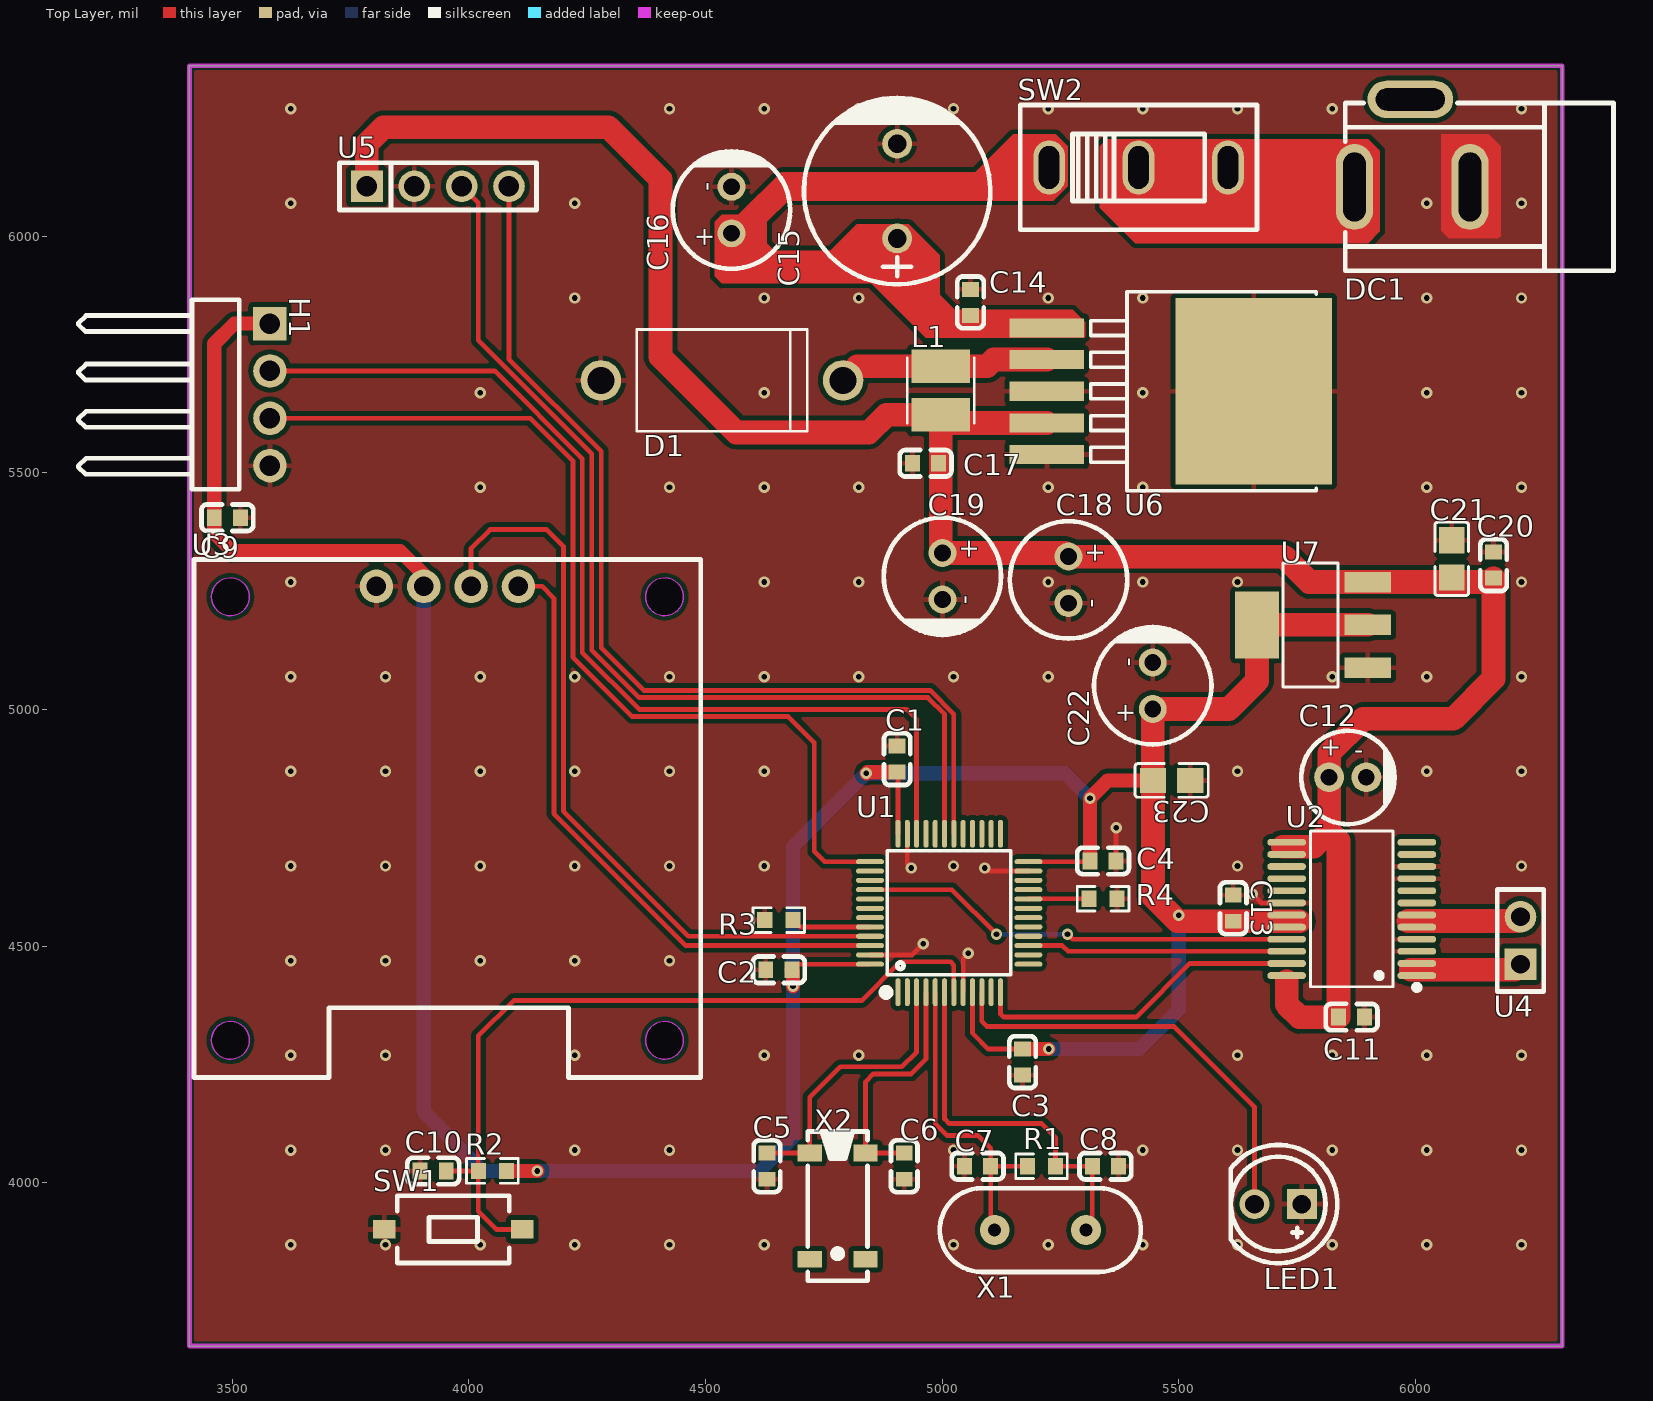
[diagram p0: Top Layer view]
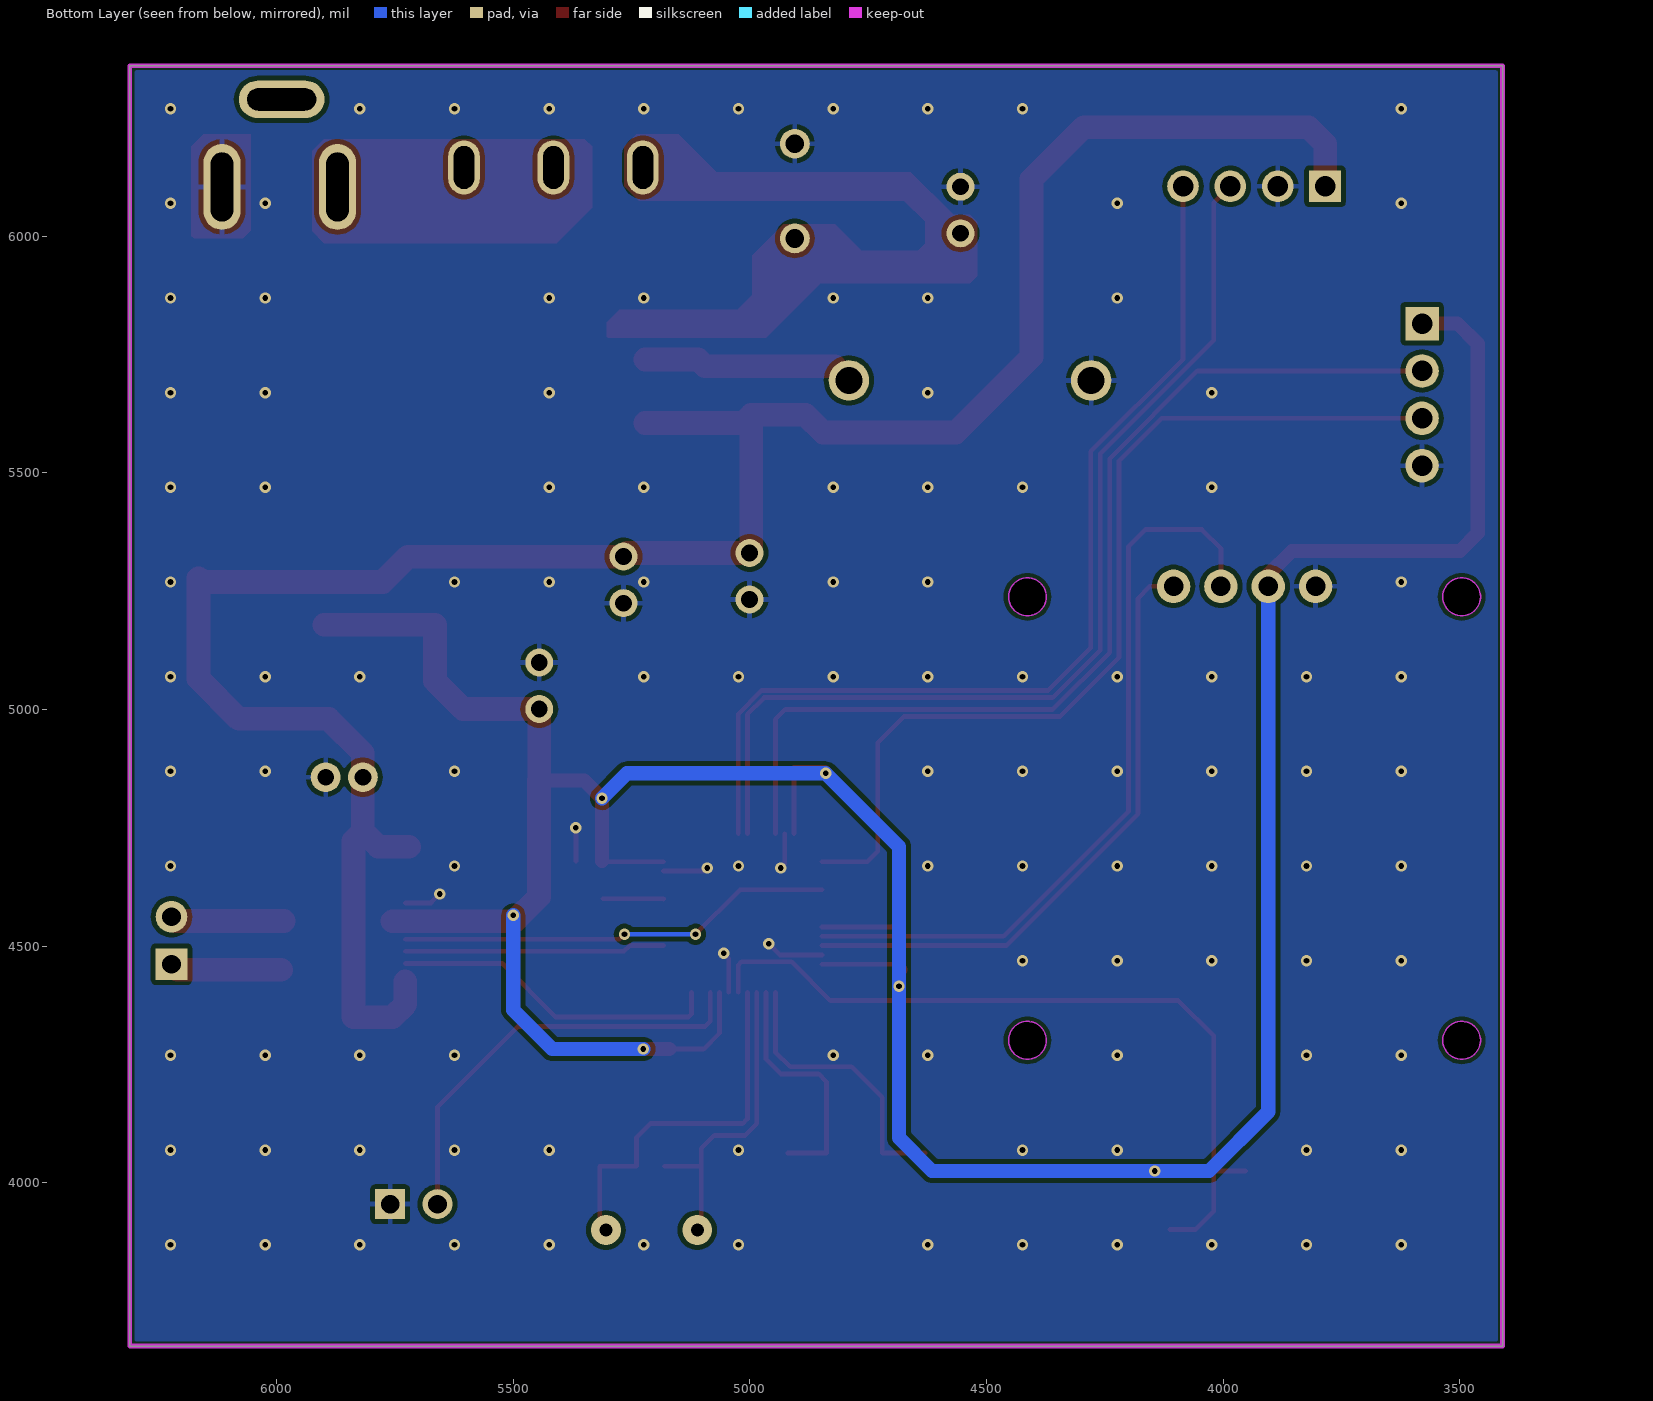
[diagram p1: Bottom Layer view, seen from below]
# Altium PCB MISC51997.pcbdoc
Units mil, origin at the board's own origin, x right, y up, seen from the top; angles counter-clockwise.
Board outline 2900 x 2705 mil, 2 copper layers (Top Layer, Bottom Layer), stack 62.206 mil thick; 43 components, 48 nets, 170 pads, 122 vias.

## Layer stack, top to bottom
Top Solder Mask Layer: solder mask 0.394, Dk 3.3
Top Layer: signal copper 1.379
Dielectric1: surface 59.449, FR4, Dk 4.5
Bottom Layer: signal copper 1.378
Bottom Solder Mask Layer: solder mask 0.394, Dk 3.3

## Board outline
3410,6360 3410,3655 6310,3655 6310,6360

## Design rules (kind name [scope] priority, off if disabled: settings)
BoardOutlineClearance copperThickness2oz_1 [All] p2 off: genericclearance=7.99 ignorepadtopadclearanceinfootprint=FALSE except(0: Arc-SplitContinuation Track-SplitContinuation SMDPad-SplitContinuation THPad-SplitContinuation Via-SplitContinuation Fill-SplitContinuation Region-SplitContinuation Poly-SplitContinuation Text-SplitContinuation Hole-SplitContinuation; 5.98: Arc-CutoutEdge SMDPad-CutoutEdge THPad-CutoutEdge Via-CutoutEdge Fill-CutoutEdge Region-CutoutEdge Text-CutoutEdge; 6.93: Hole-OutlineEdge Hole-CutoutEdge; 10: Poly-OutlineEdge Poly-CutoutEdge; 11.81: Arc-OutlineEdge Track-OutlineEdge SMDPad-OutlineEdge THPad-OutlineEdge Via-OutlineEdge Fill-OutlineEdge Region-OutlineEdge Text-OutlineEdge Track-CutoutEdge)
BoardOutlineClearance copperThickness1oz_1 [All] p4: genericclearance=4.02 ignorepadtopadclearanceinfootprint=FALSE except(0: Arc-SplitContinuation Track-SplitContinuation SMDPad-SplitContinuation THPad-SplitContinuation Via-SplitContinuation Fill-SplitContinuation Region-SplitContinuation Poly-SplitContinuation Text-SplitContinuation Hole-SplitContinuation; 6: SMDPad-CutoutEdge THPad-CutoutEdge Via-CutoutEdge Fill-CutoutEdge Region-CutoutEdge Text-CutoutEdge; 6.93: Hole-OutlineEdge Hole-CutoutEdge; 10: Poly-OutlineEdge Poly-CutoutEdge; 11.8: Arc-OutlineEdge Track-OutlineEdge SMDPad-OutlineEdge THPad-OutlineEdge Via-OutlineEdge Fill-OutlineEdge Region-OutlineEdge Text-OutlineEdge; 11.81: Arc-CutoutEdge Track-CutoutEdge)
Clearance copperThickness2oz [All] p1 off: gap=7.99 ignorepadtopadclearanceinfootprint=FALSE except(5.98: SMDPad-Track SMDPad-SMDPad THPad-Track SMDPad-THPad THPad-THPad Track-Via SMDPad-Via THPad-Via Via-Via Fill-Track Region-Track Fill-SMDPad Region-SMDPad Fill-THPad Region-THPad Fill-Via Region-Via Fill-Fill Fill-Region Region-Region Arc-Track Arc-SMDPad Arc-THPad Arc-Via Fill-Arc Region-Arc Arc-Arc Text-Track SMDPad-Text Text-THPad Text-Via Fill-Text Region-Text Arc-Text Text-Text; 6.93: Hole-Track Hole-SMDPad Hole-THPad Hole-Via Fill-Hole Region-Hole Hole-Arc Hole-Text; 10: Poly-Track Poly-SMDPad Poly-THPad Poly-Via Poly-Fill Poly-Region Poly-Poly Poly-Arc Poly-Text Poly-Hole)
Clearance copperThickness1oz [All] p3: gap=4.02 ignorepadtopadclearanceinfootprint=FALSE except(5.98: SMDPad-Track SMDPad-SMDPad THPad-Track SMDPad-THPad THPad-THPad Track-Via SMDPad-Via THPad-Via Via-Via Fill-Track Region-Track Fill-SMDPad Region-SMDPad Fill-THPad Region-THPad Fill-Via Region-Via Fill-Fill Fill-Region Region-Region; 6: Arc-Track Arc-SMDPad Arc-THPad Arc-Via Fill-Arc Region-Arc Arc-Arc Text-Track SMDPad-Text Text-THPad Text-Via Fill-Text Region-Text Arc-Text Text-Text; 6.93: Hole-Track Hole-SMDPad Hole-THPad Hole-Via Fill-Hole Region-Hole Hole-Arc Hole-Text; 10: Poly-Track Poly-SMDPad Poly-THPad Poly-Via Poly-Fill Poly-Region Poly-Poly Poly-Arc Poly-Text Poly-Hole)
Creepage creepage [All] p1: checkdistance=0 ignoreinternallayers=TRUE applytopolygonpour=TRUE
DiffPairsRouting differentialPair [All] p1: maxlimit=6 minlimit=6 mostfreqgap=6 toplayer_minwidth=5 toplayer_prefwidth=10 toplayer_maxwidth=100 toplayer_mingap=6 toplayer_prefgap=6 toplayer_maxgap=6 bottomlayer_minwidth=5 bottomlayer_prefwidth=10 bottomlayer_maxwidth=100 bottomlayer_mingap=6 bottomlayer_prefgap=6 bottomlayer_maxgap=6 maxuncoupledlength=10
HoleToHoleClearance otherClearance [All] p1: gap=11.81 allowstackedmicrovias=TRUE
Length netLength [All] p1: minlimit=0 maxlimit=0
MatchedLengths netLengthTolerance [All] p1: tolerance=1000
PasteMaskExpansion pasteMaskExpansion [All] p1: expansion=0
PlaneConnect innerPlane [All] p1: planeconnectstyle=Relief reliefexpansion=20 reliefentries=4 reliefconductorwidth=10 reliefairgap=10
PolygonConnect copperRegion [(InNet('GND'))] p1: connectstyle=Relief reliefconductorwidth=10 reliefentries=4 polygonreliefangle="90 Angle" airgapwidth=10 via.connectstyle=Relief via.reliefconductorwidth=10 via.reliefentries=4 via.polygonreliefangle="90 Angle" via.airgapwidth=10
RoutingVias viaSize [All] p1: holewidth=12.01 width=24.02 viastyle="Through Hole" minholewidth=11.81 minwidth=19.68 maxholewidth=248.03 maxwidth=393.7
SolderMaskExpansion solderMaskExpansion [IsVia] p1: expansion=-1000 istentingtop=TRUE
SolderMaskExpansion solderMaskExpansion [All] p2: expansion=2 istentingtop=FALSE
Width copperThickness2oz_2 [All] p1 off: maxlimit=100 minlimit=8 preferedwidth=10
Width copperThickness1oz_2 [All] p2: maxlimit=100 minlimit=5 preferedwidth=10

## Components (designator, comment, footprint, x,y, rotation, side; value= is the part's Value field where it differs from the comment)
C1 "100nF" C0603 4905,4895 r270 top
C2 "100nF" C0603 4655,4450 r0 top
C3 "100nF" C0603 5170,4255 r90 top
C4 "100nF" C0603 5340,4680 r180 top
C5 "20pF" C0603 4630,4035 r270 top
C6 "20pF" C0603 4920,4035 r270 top
C7 "20pF" C0603 5075,4035 r180 top
C8 "20pF" C0603 5345,4035 r0 top
C9 "100nF" C0603 3490,5405 r180 top
C10 "1uF" C0603 3925,4025 r0 top
C11 "100nF" C0603 5865,4350 r180 top
C12 "10uF" CAP-TH_BD5.0-P2.00-D0.5-FD-A 5856.9,4856.84 r0 top
C13 "100nF" C0603 5615,4580 r270 top
C14 "100nF" C0603 5060,5860 r270 top
C15 "220uF" CAP-TH_BD10.0-P5.00-D1.0-FD 4905,6095 r90 top
C16 "100uF" CAP-TH_BD6.3-P2.50-D0.5-FD 4555,6055 r90 top
C17 "100nF" C0603 4965,5520 r0 top
C18 "220uF" CAP-TH_BD6.3-P2.50-D0.5-FD_DXW025M227E112S1AA 5267.14,5273.67 r270 top
C19 "100uF" CAP-TH_BD6.3-P2.50-D0.5-FD 5000.64,5281.38 r270 top
C20 "100nF" C0603 6165,5305 r270 top
C21 "10uF" C0805 6076.65,5317.95 r270 top
C22 "100uF" CAP-TH_BD6.3-P2.50-D0.5-FD 5445,5050 r90 top
C23 "10uF" C0805 5485,4850 r180 top
D1 "1N5824" DO-201AD_BD5.3-L9.0-P13.00-D1.3-RD 4535,5695 r180 top
DC1 "DC005" DC-IN-TH_DC005 5993.2,6196.3 r180 top
H1 "PZ254R-11-04P" HDR-TH_4P-P2.54-H-M-W10.4 3580,5665 r270 top
L1 "33uH" IND-SMD_L3.5-W3.0 4997.14,5673.67 r90 top
LED1 "BL-BUB1V4V-AT" LED-TH_BD5.8-P2.54-FD_RED 5710,3955 r180 top
R1 "1MΩ" R0603 5210,4035 r180 top
R2 "10kΩ" R0603 4050,4025 r0 top
R3 "100kΩ" R0603 4655,4555 r0 top
R4 "100kΩ" R0603 5340,4600 r180 top
SW1 "TS-1101-C-W" SW-SMD_L6.0-W3.3-LS8.0_TS-1101-C-W 3967.28,3901.5 r0 top
SW2 "SS12D10G4" SW-TH_3P-P4.80-HX-SS12D10G4 5415.01,6145.01 r0 top
U1 "STM32F103C8T6" LQFP-48_L7.0-W7.0-P0.50-LS9.0-BL 5015,4570 r0 top
U2 "TB6612FNG" SSOP-24_L8.4-W5.8-P0.65-LS7.8-BL 5865.4,4578.48 r90 top
U3 "HS96L03W2C03" OLED-TH_L27.8-W27.2-P2.54_C9900033791 3955,5260 r0 top
U4 "2.54-1*2P母" HDR-TH_2P-P2.54-V-F 6221.9,4511.84 r90 top
U5 "2.54-1*4P母" HDR-TH_4P-P2.54-V-F 3935,6105 r0 top
U6 "LM2596SX-5.0-JSM" TO-263-5_L10.0-W8.4-P1.70-LS15.3-BR 5439.86,5672.17 r180 top
U7 "AMS1117-3.3" SOT-223-3_L6.5-W3.4-P2.30-LS7.0-BR 5782.28,5178.58 r0 top
X1 "8MHz" OSC-TH_L10.0-W4.5-P5.00 5207.58,3900.2 r90 top
X2 "32.768kHz" MC-306_4P-L8.0-W3.2-P5.5-BL 4779.33,3950.67 r270 top

## Footprints (in the part's own frame and the unit in brackets; to place one, negate y for a bottom-side part, rotate by r counter-clockwise, add the part's x,y. Pads: shape width x height; smd on the part's side, far side on the other; paste and mask are expansions set on the pad)
C0603 [mm]
  rect 0.8x0.9 smd: 1(-0.7,0) 2(0.7,0)
  silkscreen extent -1.39,-0.71 1.39,0.71
C0805 [mm]
  rect 1.41x1.35 smd paste-100 mask+0.051: 1(-1,0) 2(1,0)
  silkscreen extent -1.96,-0.9 1.96,0.9
CAP-TH_BD5.0-P2.00-D0.5-FD-A [mm]
  round 1.6 hole 0.9 paste+0 mask+0.05: 1(-1,0) 2(1,0)
  silkscreen extent -2.49,-2.52 2.6,2.49
CAP-TH_BD6.3-P2.50-D0.5-FD [mm]
  round 1.5 hole 0.9 paste+0 mask+0.05: 1(-1.25,0) 2(1.25,0)
  silkscreen extent -3.15,-3.15 3.21,3.15
CAP-TH_BD6.3-P2.50-D0.5-FD_DXW025M227E112S1AA [mm]
  round 1.5 hole 0.9 paste+0 mask+0.05: 1(-1.25,0) 2(1.25,0)
  silkscreen extent -3.15,-3.15 3.15,3.15
CAP-TH_BD10.0-P5.00-D1.0-FD [mm]
  round 1.6 hole 1: 1(-2.54,0) 2(2.54,0)
  silkscreen extent -5,-5 5.08,5
DC-IN-TH_DC005 [mm]
  oval 2x4.6 hole 1.2 slot 3.7 at 90 deg: 1(3.1,2.35) 2(-3.1,2.35)
  oval 4.6x2 hole 1.2 slot 3.7 at 0 deg: 3(0.1,-2.35)
  silkscreen extent -10.8,-2.15 3.6,6.85
DO-201AD_BD5.3-L9.0-P13.00-D1.3-RD [mm]
  round 2.175 hole 1.45: 1(-6.5,0) 2(6.5,0)
  silkscreen extent -4.58,-2.73 4.58,2.73
HDR-TH_2P-P2.54-V-F [mm]
  rect 1.7x1.7 hole 1: 1(-1.27,0)
  round 1.7 hole 1: 2(1.27,0)
  silkscreen extent -2.74,-1.25 2.74,1.25
HDR-TH_4P-P2.54-H-M-W10.4 [mm]
  rect 1.8x1.8 hole 1.1: 1(-3.81,0)
  round 1.8 hole 1.1: 2(-1.27,0) 3(1.27,0) 4(3.81,0)
  silkscreen extent -5.09,-10.27 5.07,-1.65
HDR-TH_4P-P2.54-V-F [mm]
  rect 1.7x1.7 hole 1.1: 1(-3.81,0)
  round 1.7 hole 1.1: 2(-1.27,0) 3(1.27,0) 4(3.81,0)
  silkscreen extent -5.29,-1.27 5.29,1.27
IND-SMD_L3.5-W3.0 [mm]
  rect 1.8x3.12 smd: 1(1.303,0) 2(-1.303,0)
  silkscreen extent -1.75,-1.8 1.75,1.8
LED-TH_BD5.8-P2.54-FD_RED [mm]
  rect 1.6x1.6 hole 1: 1(-1.27,0)
  round 1.6 hole 1: 2(1.27,0)
  silkscreen extent -3.17,-3.17 2.54,3.17
LQFP-48_L7.0-W7.0-P0.50-LS9.0-BL [mm]
  oval 0.27x1.5 smd paste+0 mask+0.05: 1(-2.75,-4.25) 2(-2.25,-4.25) 3(-1.75,-4.25) 4(-1.25,-4.25) 5(-0.75,-4.25) 6(-0.25,-4.25) 7(0.25,-4.25) 8(0.75,-4.25) 9(1.25,-4.25) 10(1.75,-4.25) 11(2.25,-4.25) 12(2.75,-4.25) 25(2.75,4.25) 26(2.25,4.25) 27(1.75,4.25) 28(1.25,4.25) 29(0.75,4.25) 30(0.25,4.25) 31(-0.25,4.25) 32(-0.75,4.25) 33(-1.25,4.25) 34(-1.75,4.25) 35(-2.25,4.25) 36(-2.75,4.25)
  oval 1.5x0.27 smd paste+0 mask+0.05: 13(4.25,-2.75) 14(4.25,-2.25) 15(4.25,-1.75) 16(4.25,-1.25) 17(4.25,-0.75) 18(4.25,-0.25) 19(4.25,0.25) 20(4.25,0.75) 21(4.25,1.25) 22(4.25,1.75) 23(4.25,2.25) 24(4.25,2.75) 37(-4.25,2.75) 38(-4.25,2.25) 39(-4.25,1.75) 40(-4.25,1.25) 41(-4.25,0.75) 42(-4.25,0.25) 43(-4.25,-0.25) 44(-4.25,-0.75) 45(-4.25,-1.25) 46(-4.25,-1.75) 47(-4.25,-2.25) 48(-4.25,-2.75)
  silkscreen extent -3.59,-4.46 3.3,3.34
MC-306_4P-L8.0-W3.2-P5.5-BL [mm]
  rect 0.9x1.3 smd: 1(-2.85,-1.5) 2(2.85,-1.5) 3(2.85,1.5) 4(-2.85,1.5)
  silkscreen extent -4,-1.6 4,1.6
OLED-TH_L27.8-W27.2-P2.54_C9900033791 [mm]
  round 1.8 hole 1.05 paste+0 mask+0.05: 1(-3.81,0) 2(-1.27,0) 3(1.27,0) 4(3.81,0)
  Board Outline Layer circle w0.003: c-11.65,-0.56 r1.016
  Board Outline Layer circle w0.003: c11.65,-0.56 r1.016
  Board Outline Layer circle w0.003: c-11.65,-24.36 r1.016
  Board Outline Layer circle w0.003: c11.65,-24.36 r1.016
  Board Outline Layer region: -10.634,-0.56 -10.735,-1.001 -11.016,-1.354 -11.424,-1.551 -11.876,-1.551 -12.283,-1.354 -12.565,-1.001 -12.666,-0.56 -12.666,-0.56 -12.565,-0.119 -12.283,0.234 -11.876,0.431 -11.424,0.431 -11.016,0.234 -10.735,-0.119 -10.634,-0.56
  Board Outline Layer region: -10.634,-0.56 -10.643,-0.698 -10.672,-0.834 -10.718,-0.965 -10.782,-1.088 -10.862,-1.201 -10.956,-1.303 -11.064,-1.39 -11.183,-1.462 -11.31,-1.517 -11.443,-1.555 -11.581,-1.574 -11.719,-1.574 -11.857,-1.555 -11.99,-1.517 -12.117,-1.462 -12.236,-1.39 -12.343,-1.303 -12.438,-1.201 -12.518,-1.088 -12.582,-0.965 -12.628,-0.834 -12.656,-0.698 -12.666,-0.56 -12.656,-0.422 -12.628,-0.286 -12.582,-0.155 -12.518,-0.032 -12.438,0.081 -12.343,0.183 -12.236,0.27 -12.117,0.342 -11.99,0.397 -11.857,0.435 -11.719,0.454 -11.581,0.454 -11.443,0.435 -11.31,0.397 -11.183,0.342 -11.064,0.27 -10.956,0.183 -10.862,0.081 -10.782,-0.032 -10.718,-0.155 -10.672,-0.286 -10.643,-0.422
  Board Outline Layer region: 12.666,-0.56 12.565,-1.001 12.283,-1.354 11.876,-1.551 11.424,-1.551 11.017,-1.354 10.735,-1.001 10.634,-0.56 10.634,-0.56 10.735,-0.119 11.017,0.234 11.424,0.431 11.876,0.431 12.283,0.234 12.565,-0.119 12.666,-0.56
  Board Outline Layer region: 12.666,-0.56 12.657,-0.698 12.628,-0.834 12.582,-0.965 12.518,-1.088 12.438,-1.201 12.343,-1.303 12.236,-1.39 12.117,-1.462 11.99,-1.517 11.857,-1.555 11.719,-1.574 11.581,-1.574 11.443,-1.555 11.31,-1.517 11.183,-1.462 11.064,-1.39 10.957,-1.303 10.862,-1.201 10.782,-1.088 10.718,-0.965 10.672,-0.834 10.643,-0.698 10.634,-0.56 10.643,-0.422 10.672,-0.286 10.718,-0.155 10.782,-0.032 10.862,0.081 10.957,0.183 11.064,0.27 11.183,0.342 11.31,0.397 11.443,0.435 11.581,0.454 11.719,0.454 11.857,0.435 11.99,0.397 12.117,0.342 12.236,0.27 12.343,0.183 12.438,0.081 12.518,-0.032 12.582,-0.155 12.628,-0.286 12.657,-0.422
  Board Outline Layer region: -10.634,-24.36 -10.735,-24.801 -11.016,-25.154 -11.424,-25.35 -11.876,-25.35 -12.283,-25.154 -12.565,-24.801 -12.666,-24.36 -12.666,-24.36 -12.565,-23.919 -12.283,-23.566 -11.876,-23.369 -11.424,-23.369 -11.016,-23.566 -10.735,-23.919 -10.634,-24.36
  Board Outline Layer region: -10.634,-24.36 -10.643,-24.498 -10.672,-24.634 -10.718,-24.765 -10.782,-24.888 -10.862,-25.001 -10.956,-25.102 -11.064,-25.19 -11.183,-25.262 -11.31,-25.317 -11.443,-25.355 -11.581,-25.374 -11.719,-25.374 -11.857,-25.355 -11.99,-25.317 -12.117,-25.262 -12.236,-25.19 -12.343,-25.102 -12.438,-25.001 -12.518,-24.888 -12.582,-24.765 -12.628,-24.634 -12.656,-24.498 -12.666,-24.36 -12.656,-24.222 -12.628,-24.086 -12.582,-23.955 -12.518,-23.832 -12.438,-23.719 -12.343,-23.617 -12.236,-23.53 -12.117,-23.458 -11.99,-23.403 -11.857,-23.365 -11.719,-23.346 -11.581,-23.346 -11.443,-23.365 -11.31,-23.403 -11.183,-23.458 -11.064,-23.53 -10.956,-23.617 -10.862,-23.719 -10.782,-23.832 -10.718,-23.955 -10.672,-24.086 -10.643,-24.222
  Board Outline Layer region: 12.666,-24.36 12.565,-24.801 12.283,-25.154 11.876,-25.35 11.424,-25.35 11.017,-25.154 10.735,-24.801 10.634,-24.36 10.634,-24.36 10.735,-23.919 11.017,-23.566 11.424,-23.369 11.876,-23.369 12.283,-23.566 12.565,-23.919 12.666,-24.36
  Board Outline Layer region: 12.666,-24.36 12.657,-24.498 12.628,-24.634 12.582,-24.765 12.518,-24.888 12.438,-25.001 12.343,-25.102 12.236,-25.19 12.117,-25.262 11.99,-25.317 11.857,-25.355 11.719,-25.374 11.581,-25.374 11.443,-25.355 11.31,-25.317 11.183,-25.262 11.064,-25.19 10.957,-25.102 10.862,-25.001 10.782,-24.888 10.718,-24.765 10.672,-24.634 10.643,-24.498 10.634,-24.36 10.643,-24.222 10.672,-24.086 10.718,-23.955 10.782,-23.832 10.862,-23.719 10.957,-23.617 11.064,-23.53 11.183,-23.458 11.31,-23.403 11.443,-23.365 11.581,-23.346 11.719,-23.346 11.857,-23.365 11.99,-23.403 12.117,-23.458 12.236,-23.53 12.343,-23.617 12.438,-23.719 12.518,-23.832 12.582,-23.955 12.628,-24.086 12.657,-24.222
  Multi-Layer board cut-out: -10.634,-0.56 -10.735,-1.001 -11.016,-1.354 -11.424,-1.551 -11.876,-1.551 -12.283,-1.354 -12.565,-1.001 -12.666,-0.56 -12.666,-0.56 -12.565,-0.119 -12.283,0.234 -11.876,0.431 -11.424,0.431 -11.016,0.234 -10.735,-0.119 -10.634,-0.56
  Multi-Layer board cut-out: 12.666,-0.56 12.565,-1.001 12.283,-1.354 11.876,-1.551 11.424,-1.551 11.017,-1.354 10.735,-1.001 10.634,-0.56 10.634,-0.56 10.735,-0.119 11.017,0.234 11.424,0.431 11.876,0.431 12.283,0.234 12.565,-0.119 12.666,-0.56
  Multi-Layer board cut-out: -10.634,-24.36 -10.735,-24.801 -11.016,-25.154 -11.424,-25.35 -11.876,-25.35 -12.283,-25.154 -12.565,-24.801 -12.666,-24.36 -12.666,-24.36 -12.565,-23.919 -12.283,-23.566 -11.876,-23.369 -11.424,-23.369 -11.016,-23.566 -10.735,-23.919 -10.634,-24.36
  Multi-Layer board cut-out: 12.666,-24.36 12.565,-24.801 12.283,-25.154 11.876,-25.35 11.424,-25.35 11.017,-25.154 10.735,-24.801 10.634,-24.36 10.634,-24.36 10.735,-23.919 11.017,-23.566 11.424,-23.369 11.876,-23.369 12.283,-23.566 12.565,-23.919 12.666,-24.36
  silkscreen extent -13.6,-26.36 13.6,1.44
OSC-TH_L10.0-W4.5-P5.00 [mm]
  round 1.6 hole 0.7: 1(0,2.45) 2(0,-2.45)
  silkscreen extent -2.25,-5.39 2.25,5.39
R0603 [mil]
  rect 31.75x34.02 smd paste-3937.01 mask+2: 1(-29.66,0) 2(29.66,0)
  silkscreen extent -55,-26 55,26
SOT-223-3_L6.5-W3.4-P2.30-LS7.0-BR [mm]
  rect 2.5x1.1 smd: 1(2.97,-2.3) 2(2.97,0) 3(2.97,2.3)
  rect 2.34x3.6 smd: 4(-2.97,0)
  silkscreen extent -1.57,-3.33 1.37,3.33
SSOP-24_L8.4-W5.8-P0.65-LS7.8-BL [mil]
  oval 14.33x81.97 smd: 1(-140.75,-137.44) 2(-115.16,-137.44) 3(-89.57,-137.44) 4(-63.98,-137.44) 5(-38.39,-137.44) 6(-12.79,-137.44) 7(12.8,-137.44) 8(38.39,-137.44) 9(63.98,-137.44) 10(89.57,-137.44) 11(115.16,-137.44) 12(140.75,-137.44) 13(140.75,137.44) 14(115.16,137.44) 15(89.57,137.44) 16(63.98,137.44) 17(38.39,137.44) 18(12.8,137.44) 19(-12.79,137.44) 20(-38.39,137.44) 21(-63.98,137.44) 22(-89.57,137.44) 23(-115.16,137.44) 24(-140.75,137.44)
  silkscreen extent -172,-143 164,87
SW-SMD_L6.0-W3.3-LS8.0_TS-1101-C-W [mm]
  rect 1.2x1 smd: 1(-3.7,0) 2(3.7,0)
  silkscreen extent -3,-1.8 3,1.8
SW-TH_3P-P4.80-HX-SS12D10G4 [mm]
  oval 1.7x2.9 hole 1.1 slot 2.3 at 90 deg paste+0 mask+0.05: 1(-4.8,0) 2(0,0) 3(4.8,0)
  silkscreen extent -6.35,-3.35 6.35,3.35
TO-263-5_L10.0-W8.4-P1.70-LS15.3-BR [mm]
  rect 4x1.02 smd: 1(5.55,-3.4) 2(5.55,-1.7) 3(5.55,0) 4(5.55,1.7) 5(5.55,3.4)
  rect 8.4x10 smd: 6(-5.55,0)
  silkscreen extent -8.91,-5.33 3.2,5.33

## Via types
v1: diameter 24.02, hole 12, Top Layer to Bottom Layer, 122 vias

## Nets (pads, with @x,y where several pads share a name; then routed paths per layer and width w, separated by ;. In a path a pad name is that pad's centre, name@x,y a point inside that pad or via, vN(x,y) a via of type N, cw(c..) or ccw(c..) an arc to the next point about the centre after c; other vN are vias at no path point)
$1N2: DC1.1 SW2.2 SW2.3
$1N10: D1.1 L1.1 U6.2 | length 448.7
  Top Layer w50: D1.1 4820.88,5724.97 L1.1 5094.97,5724.97 5109.1,5739.1 U6.2
+5V: C11.2 C12.1 C17.2 C18.1 C19.1 C20.2 C21.2 L1.2 U2.13 U2.14 U2.24 U5.1 U6.4 U7.3 | length 5007.8
  Top Layer w50: U5.1 3784.64,6105.36 3784.64,6194.64 3820,6230 4295,6230 4405,6120 4405,5745 4565,5585 4845,5585 4882.37,5622.37 L1.2 ; U6.4 5014.27,5605.24 L1.2 ; 5720,4710 5785,4710 5817.53,4742.53 ; 5727.96,4425.18 5727.96,4377.04 5755,4350 C11.2 5837.44,4722.63 5817.53,4742.53 ; L1.2 4997.14,5334.09 C19.1 5259.43,5330.59 C18.1 5722.12,5322.88 5775.87,5269.13 U7.3 6156.69,5269.13 C20.2 6165,5065 6080,4980 5890,4980 5817.53,4907.53 C12.1 5817.53,4742.53
AO1: U2.1 U2.2 U4.1 | length 236.8
  Top Layer w50: 5990,4450 6210.07,4450 U4.1
AO2: U2.5 U2.6 U4.2 | length 240.5
  Top Layer w50: 5985,4553.14 6213.2,4553.14 U4.2
BAT: C14.2 C15.1 C16.1 SW2.1 U6.1
BOOT0: R3.2 U1.44 | length 169
  Top Layer w10: R3.2 4699.19,4540.47 U1.44
BOOT1: R4.2 U1.20 | length 128.2
  Top Layer w10: U1.20 5182.79,4600 R4.2
GND: C1.1 C2.1 C3.1 C4.1 C5.2 C6.2 C7.2 C8.2 C9.1 C10.1 C11.1 C12.2 C13.1 C14.1 C15.2 C16.2 C17.1 C18.2 C19.2 C20.1 C21.1 C22.2 C23.1 D1.2 DC1.2 H1.4 LED1.1 R3.1 R4.1 SW1.1 U1.8 U1.23 U1.35 U1.47 U2.3 U2.4 U2.9 U2.10 U2.18 U3.1 U5.2 U6.3 U6.5 U6.6 U7.1 | length 530.3
  Top Layer w10: U1.47 4936.42,4481.42 v1(4960,4505) ; U1.35 4926.42,4673.58 v1(4935,4665) ; U1.8 5044.53,4474.53 v1(5055,4485) ; v1(5090,4665) 5096.42,4658.58 U1.23 ; C4.1 v1(5367.56,4750) ; v1(5655,4610) 5673.72,4591.28 U2.18
  other v1: 3624.1,3869.1 3824.1,3869.1 4024.1,3869.1 4224.1,3869.1 4424.1,3869.1 4624.1,3869.1 5024.1,3869.1 5224.1,3869.1 5424.1,3869.1 5624.1,3869.1 5824.1,3869.1 6024.1,3869.1 6224.1,3869.1 3624.1,4069.1 3824.1,4069.1 4224.1,4069.1 4424.1,4069.1 5024.1,4069.1 5424.1,4069.1 5624.1,4069.1 5824.1,4069.1 6024.1,4069.1 6224.1,4069.1 3624.1,4269.1 3824.1,4269.1 4224.1,4269.1 4624.1,4269.1 4824.1,4269.1 5624.1,4269.1 5824.1,4269.1 6024.1,4269.1 6224.1,4269.1 3624.1,4469.1 3824.1,4469.1 4024.1,4469.1 4224.1,4469.1 4424.1,4469.1 3624.1,4669.1 3824.1,4669.1 4024.1,4669.1 4224.1,4669.1 4424.1,4669.1 4624.1,4669.1 5024.1,4669.1 5624.1,4669.1 6224.1,4669.1 3624.1,4869.1 3824.1,4869.1 4024.1,4869.1 4224.1,4869.1 4424.1,4869.1 4624.1,4869.1 5624.1,4869.1 6024.1,4869.1 6224.1,4869.1 3624.1,5069.1 3824.1,5069.1 4024.1,5069.1 4224.1,5069.1 4424.1,5069.1 4624.1,5069.1 4824.1,5069.1 5024.1,5069.1 5224.1,5069.1 5824.1,5069.1 6024.1,5069.1 6224.1,5069.1 3624.1,5269.1 4624.1,5269.1 4824.1,5269.1 5224.1,5269.1 5424.1,5269.1 5624.1,5269.1 6224.1,5269.1 4024.1,5469.1 4424.1,5469.1 4624.1,5469.1 4824.1,5469.1 5224.1,5469.1 5424.1,5469.1 6024.1,5469.1 6224.1,5469.1 4024.1,5669.1 4624.1,5669.1 5424.1,5669.1 6024.1,5669.1 6224.1,5669.1 4224.1,5869.1 4624.1,5869.1 4824.1,5869.1 5224.1,5869.1 5424.1,5869.1 6024.1,5869.1 6224.1,5869.1 3624.1,6069.1 4224.1,6069.1 6024.1,6069.1 6224.1,6069.1 3624.1,6269.1 4424.1,6269.1 4624.1,6269.1 4824.1,6269.1 5024.1,6269.1 5224.1,6269.1 5424.1,6269.1 5624.1,6269.1 5824.1,6269.1 6224.1,6269.1
OSCIN: C7.1 R1.2 U1.5 X1.1 | length 670.4
  Top Layer w10: U1.5 4985.47,4124.53 5010,4100 5075,4100 5102.56,4072.44 C7.1 ; X1.1 5102.56,3908.77 C7.1 ; R1.2 C7.1
OSCOUT: C8.1 R1.1 U1.6 X1.2 | length 797.2
  Top Layer w10: U1.6 5005.16,4134.84 5015,4125 5210,4125 5239.66,4095.34 R1.1 C8.1 5317.44,3913.6 X1.2
PA0: LED1.2 U1.10 | length 917.7
  Top Layer w10: U1.10 5083.9,4341.1 5095,4330 5490,4330 5660,4160 LED1.2
PA1: U1.11
PA2: U1.12 U2.23 | length 700.4
  Top Layer w10: U1.12 5123.27,4356.73 5130,4350 5410,4350 5523.32,4463.32 U2.23
PA3: U1.13
PA4: U1.14
PA5: U1.15 U2.22 | length 550.7
  Top Layer w10: U1.15 5253.9,4501.1 5266.09,4488.91 U2.22
PA6: U1.16
PA7: U1.17
PA8: U1.29
PA9: U1.30 U5.4 | length 2111.4
  Top Layer w10: U5.4 4085,5740 4280,5545 4280,5130 4370,5040 4975,5040 5024.84,4990.16 U1.30
PA10: U1.31 U5.3 | length 2147.6
  Top Layer w10: U5.3 4020,6070 4020,5780 4260,5540 4260,5125 4360,5025 4970,5025 5005.16,4989.84 U1.31
PA11: U1.32
PA12: U1.33
PA15: U1.38
PB0: U1.18
PB1: U1.19
PB3: U1.39
PB4: U1.40 U2.21 | length 923.7
  Top Layer w10: U1.40 5020.79,4619.21 v1(5115,4525) ; v1(5265,4525) 5275.49,4514.51 U2.21
  Bottom Layer w10: v1(5115,4525) v1(5265,4525)
PB5: U1.41
PB6: U1.42
PB7: U1.43
PB8: U1.45 U3.3 | length 1623.2
  Top Layer w10: U3.3 4005,5340 4045,5380 4165,5380 4200,5345 4200,4785 4464.21,4520.79 U1.45
PB9: U1.46 U3.4 | length 1323.6
  Top Layer w10: U3.4 4155,5260 4180,5235 4180,4780 4458.9,4501.1 U1.46
PB10: U1.21
PB11: U1.22
PB12: U1.25
PB13: U1.26
PB14: U1.27
PB15: U1.28
PC13: U1.2
PC14: C5.1 U1.3 X2.1 | length 599.9
  Top Layer w10: C5.1 4630.31,4062.87 X2.1 4720.27,4180.27 4785,4245 4915,4245 4946.1,4276.1 U1.3
PC15: C6.1 U1.4 X2.4 | length 521.2
  Top Layer w10: C6.1 4919.69,4062.87 X2.4 4838.39,4213.39 4855,4230 4935,4230 4965.79,4260.79 U1.4
RESET: C10.2 R2.1 SW1.2 U1.7 | length 1676.5
  Top Layer w10: C10.2 R2.1 ; SW1.2 4058.5,3901.5 4020.34,3939.66 R2.1 ; U1.7 5024.84,4460 5017.77,4467.07 4912.07,4467.07 4830,4385 4095,4385 4020.34,4310.34 R2.1
SWCLK: H1.3 U1.37 | length 2033.5
  Top Layer w10: H1.3 4130,5615 4220,5525 4220,5110 4345,4985 4675,4985 4730,4930 4730,4700 4751.73,4678.27 U1.37
SWDIO: H1.2 U1.34 | length 2152.8
  Top Layer w10: H1.2 4055,5715 4240,5530 4240,5120 4360,5000 4925,5000 4946.1,4978.9 U1.34
VBAT: U1.1
VCC: C1.2 C2.2 C3.2 C4.2 C9.2 C13.2 C22.1 C23.2 H1.1 R2.2 U1.9 U1.24 U1.36 U1.48 U2.19 U2.20 U3.2 U7.2 U7.4 | length 7313.8
  Top Layer w10: C2.2 4694.29,4461.73 U1.48 ; C1.2 4906.73,4865.71 U1.36 ; U1.9 5064.21,4315.79 5097.44,4282.56 C3.2 ; U1.24 5310.71,4678.27 C4.2
  Top Layer w30: H1.1 3505,5815 3462.44,5772.44 C9.2 3462.44,5372.56 3500,5335 3855,5335 3905,5285 U3.2 ; R2.2 v1(4145,4025) ; C2.2 4685,4447.56 v1(4685,4415) ; v1(4840,4865) 4842.44,4867.44 C1.2 ; C3.2 v1(5225,4282.56) ; C4.2 v1(5312.44,4812.44) 5350,4850 C23.2
  Top Layer w50: C13.2 C13.2@5615.21,4552.65 ; 5755,4552.65 C13.2@5615.21,4552.65 ; U7.2 U7.4 5665.35,5060.35 5605.79,5000.79 C22.1 5445,4850.63 C23.2 5445.63,4604.37 5497.35,4552.65 C13.2@5615.21,4552.65
  Bottom Layer w30: U3.2 3905,4150 4030,4025 v1(4145,4025) 4615,4025 4685,4095 v1(4685,4415) 4685,4710 v1(4840,4865) 5259.88,4865 v1(5312.44,4812.44) ; v1(5225,4282.56) 5417.56,4282.56 5500,4365 v1(5500,4565)
pads on no net: DC1.3 U2.7 U2.8 U2.11 U2.12 U2.15 U2.16 U2.17 X2.2 X2.3

## Polygon pours and split planes (outlines as drawn)
GND on Top Layer (solid, remove dead copper, pour order 0): 3000,6750 3000,3000 6610,3000 6610,6750
GND on Bottom Layer (solid, remove dead copper, pour order 2): 3130,6640 3130,3100 6640,3100 6640,6640

## Keep-outs
Board Outline Layer:
  the board outline again, w10

## Other copper
Top Layer:
  region net $1N2: 5900,6205 5925,6180 5925,6010 5900,5985 5408.41,5985 5333.23,6060.18 5333.23,6189.49 5348.74,6205
  region net BAT: 5240,6215 5265,6190 5265,6105 5235,6075 4675.09,6075 4630,6029.91 4630,5985 4645.78,5969.22 4764.22,5969.22 4820,6025 4930,6025 4995,5960 4995,5876.01 5027.05,5843.97 5276.4,5843.97 5302.14,5818.23 5302.14,5787.14 5300,5785 4965,5785 4850,5900 4535,5900 4520,5915 4520,6030.78 4534.05,6044.83 4569.83,6044.83 4660,6135 5070,6135 5150,6215
  region net GND: 6054.15,6215 6155,6215 6180,6190 6180,6000 6175,5995 6070,5995 6054.15,6010.85